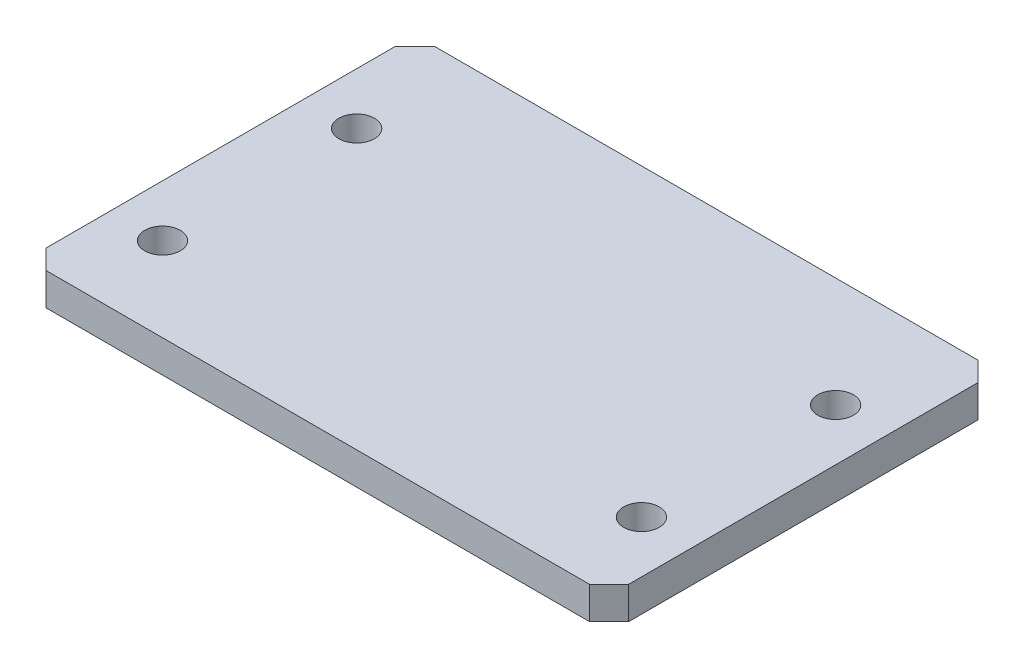
SolidWorks part; units mm, degrees
material "A6061 T6"
ref_plane "前视基准面" through (0, 0, 0) normal (0, 0, 1) x (1, 0, 0)
ref_plane "上视基准面" through (0, 0, 0) normal (0, 1, 0) x (1, 0, 0)
ref_plane "右视基准面" through (0, 0, 0) normal (1, 0, 0) x (0, 0, -1)
sketch "草图1" plane through (0, 0, 0) normal (0, 1, 0) x (1, 0, 0)
  line L1 (-45, 30) -> (45, 30)
  line L2 (-45, 30) -> (-45, -30)
  line L3 (-45, -30) -> (45, -30)
  line L4 (45, 30) -> (45, -30)
  line L5 (-45, 30) -> (45, -30) construction
  line L6 (-45, -30) -> (45, 30) construction
  point P0 (0, 0)
  dimension "D1" = 90
  dimension "D2" = 60
extrude "凸台-拉伸1" add sketch "草图1" along normal blind 5
chamfer "倒角1" distance 3 angle 45 4 edges at (-45, 2.5, -30) (45, 2.5, -30) (45, 2.5, 30) (-45, 2.5, 30)
sketch "草图2" plane through (0, 5, 0) normal (0, 1, 0) x (1, 0, 0)
  circle A0 centre (37, -17) radius 2.75
  circle A1 centre (-37, -17) radius 2.75
  circle A2 centre (37, 13) radius 2.75
  circle A3 centre (-37, 13) radius 2.75
  dimension "D1" = 5.5
extrude "切除-拉伸1" cut sketch "草图2" against normal blind 10
